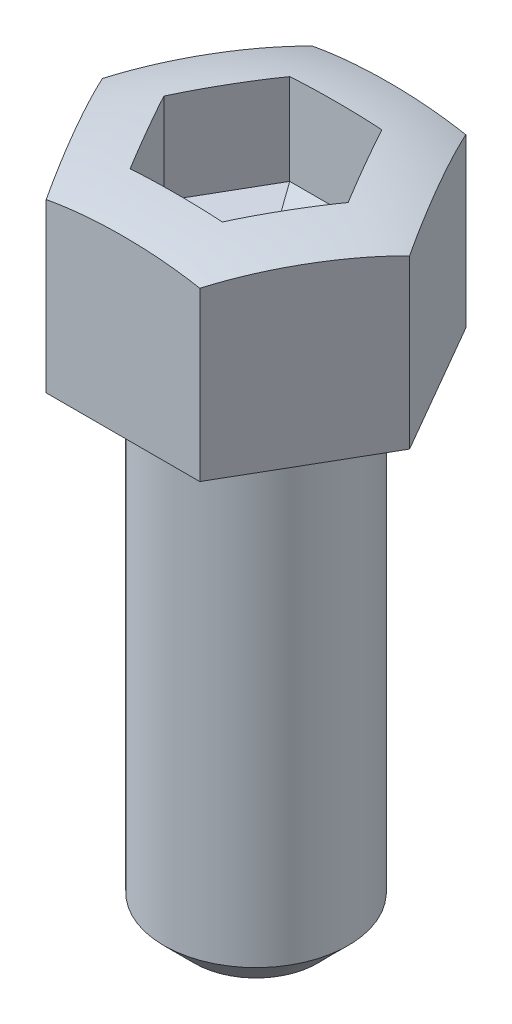
from build123d import *

# Parameters (mm, degrees)
SKETCH2_W          = 12.434421081
SKETCH2_H          = 11.052818739
CUT_EXTRUDE2_DEPTH = 6
CUT_EXTRUDE3_DEPTH = 3
CHAMFER1_SIZE      = 1


with BuildPart() as part:
    # Sketch1 → Revolve1 (revolve)
    with BuildSketch(Plane.XY, mode=Mode.PRIVATE) as revolve1_sk:
        Polygon((0, 0), (3, 0), (3, 16), (5, 16), (5, 22), (0, 22), (0, 0.812520437), align=None)
    revolve(revolve1_sk.sketch.rotate(Axis((0, 22, 0), (0, -1, 0)), 90), axis=Axis((0, 22, 0), (0, -1, 0)))

    # Sketch2 → Cut-Extrude2 (cut)
    with BuildSketch(Plane(origin=(0, 22, 0), x_dir=(1, 0, 0), z_dir=(0, 1, 0))):
        with Locations((0.708980149, -0.054536934)):
            Rectangle(SKETCH2_W, SKETCH2_H)
        Polygon((5, 0), (2.5, 4.330127019), (-2.5, 4.330127019), (-5, 0), (-2.5, -4.330127019), (2.5, -4.330127019), align=None, mode=Mode.SUBTRACT)
    extrude(amount=-CUT_EXTRUDE2_DEPTH, mode=Mode.SUBTRACT)

    # Sketch3 → Cut-Extrude3 (cut)
    with BuildSketch(Plane(origin=(0, 22, 0), x_dir=(1, 0, 0), z_dir=(0, 1, 0))):
        Polygon((3, 0), (1.5, 2.598076211), (-1.5, 2.598076211), (-3, 0), (-1.5, -2.598076211), (1.5, -2.598076211), align=None)
    extrude(amount=-CUT_EXTRUDE3_DEPTH, mode=Mode.SUBTRACT)

    # Sketch5 → Cut-Loft1 section 0
    with BuildSketch(Plane(origin=(0, 19, 0), x_dir=(1, 0, 0), z_dir=(0, 1, 0)), mode=Mode.PRIVATE) as cut_loft1_s0:
        with BuildLine():
            Line((1.5, 2.598076211), (-1.5, 2.598076211))
            Line((-1.5, 2.598076211), (-3, 0))
            Line((-3, 0), (-1.5, -2.598076211))
            Line((-1.5, -2.598076211), (1.5, -2.598076211))
            Line((1.5, -2.598076211), (3, 0))
            Line((3, 0), (1.5, 2.598076211))
        make_face()
    loft([cut_loft1_s0.sketch, Vertex(0, 17.68563071, 0)], mode=Mode.SUBTRACT)

    # Chamfer1
    chamfer1_edges = [part.edges().sort_by_distance(p)[0] for p in [
        (0, 0, -3),
    ]]
    chamfer(chamfer1_edges, length=CHAMFER1_SIZE)

    # Sketch6 → Cut-Revolve1 (revolve, cut)
    with BuildSketch(Plane(origin=(0, 0, 0), x_dir=(0, 0, -1), z_dir=(1, 0, 0)), mode=Mode.PRIVATE) as cut_revolve1_sk:
        with BuildLine():
            Line((-5.464509536, 21.264956491), (-5.887873992, 22.169745092))
            Line((-5.887873992, 22.169745092), (-3.885003272, 23.64244415))
            Line((-3.885003272, 23.64244415), (-2.598076211, 22))
            ThreePointArc((-2.598076211, 22), (-4.060125505, 21.744916236), (-5.464509536, 21.264956491))
        make_face()
    revolve(cut_revolve1_sk.sketch.rotate(Axis((0, 16, 0), (0, 1, 0)), 149.999999986), axis=Axis((0, 16, 0), (0, 1, 0)), mode=Mode.SUBTRACT)


solid = part.part
